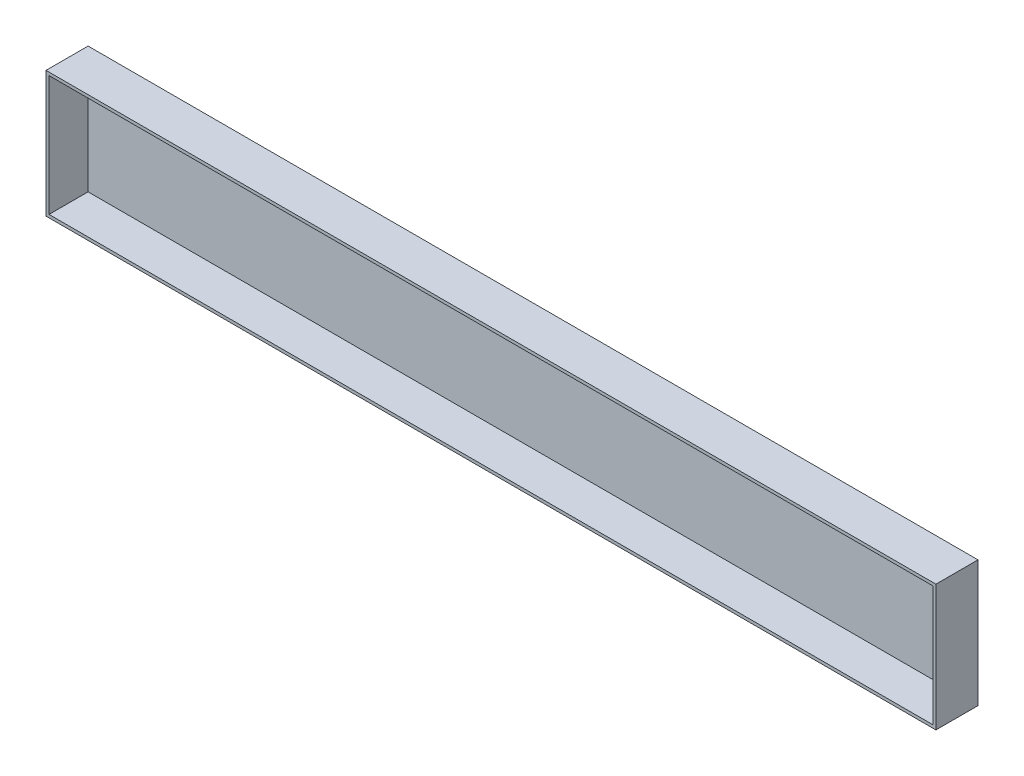
from build123d import *

# Parameters (mm, degrees)
SKETCH_1_W        = 1480
SKETCH_1_H        = 210
SKETCH_1_W_2      = 1470
SKETCH_1_H_2      = 200
EXTRUDE_1_DEPTH   = 70
SKETCH_2_W        = 5
SKETCH_2_H        = 210
EXTRUDE_1_2_DEPTH = 1470


with BuildPart() as part:
    # 草图1 → Extrude 1 (new body)
    with BuildSketch(Plane.XY):
        Rectangle(SKETCH_1_W, SKETCH_1_H)
        Rectangle(SKETCH_1_W_2, SKETCH_1_H_2, mode=Mode.SUBTRACT)
    extrude(amount=EXTRUDE_1_DEPTH)

    # 草图2 → Extrude 1 2 (add)
    with BuildSketch(Plane.ZY.offset(-735)):
        with Locations((2.5, 0)):
            Rectangle(SKETCH_2_W, SKETCH_2_H)
    extrude(amount=EXTRUDE_1_2_DEPTH)


solid = part.part
